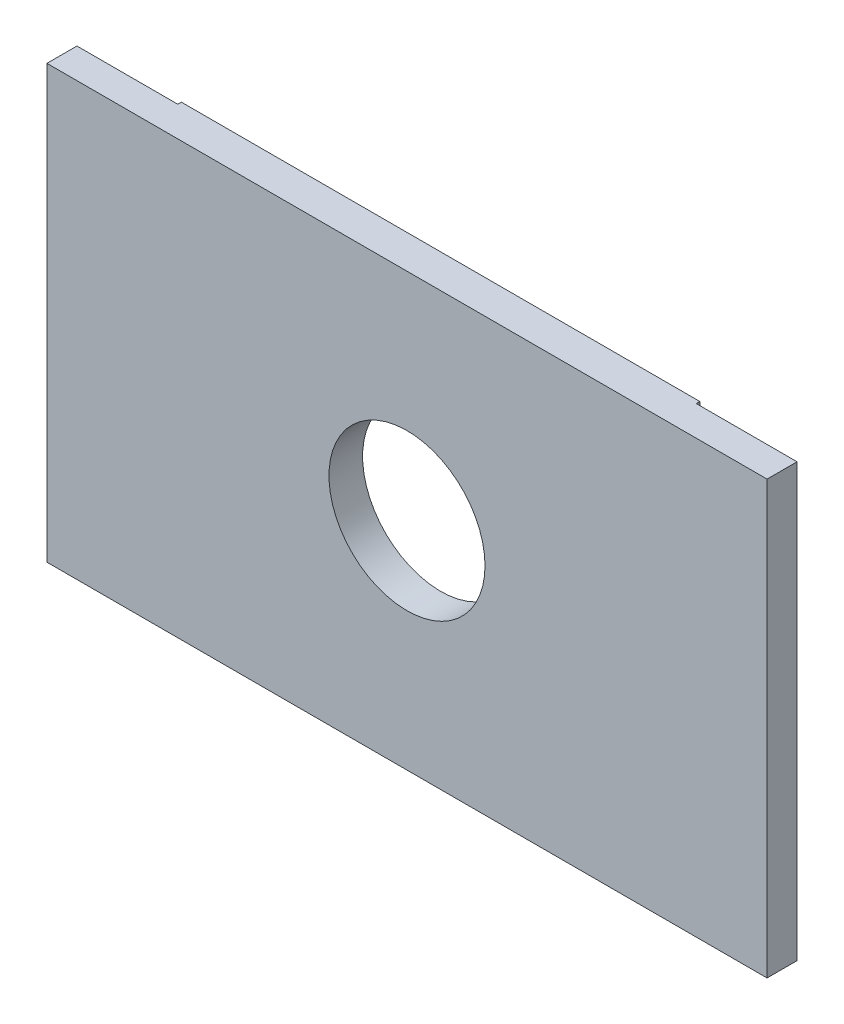
from build123d import *

# Parameters (mm, degrees)
SKETCH_1_W          = 300
SKETCH_1_H          = 180
EXTRUDE_1_DEPTH     = 14
SKETCH_2_W          = 42
SKETCH_2_H          = 180
CUT_EXTRUDE_1_DEPTH = 1.5
CUT_EXTRUDE_2_REACH = 177.488
SKETCH_3_R          = 32.5


with BuildPart() as part:
    # 草图1 → 凸台-拉伸1 (new body)
    with BuildSketch(Plane.XY):
        Rectangle(SKETCH_1_W, SKETCH_1_H)
    extrude(amount=EXTRUDE_1_DEPTH)

    # 草图2 → 切除-拉伸1 (cut)
    with BuildSketch(Plane(origin=(0, 0, 0), x_dir=(-1, 0, 0), z_dir=(0, 0, -1))):
        with Locations((129, 0)):
            Rectangle(SKETCH_2_W, SKETCH_2_H)
        with Locations((-129, 0)):
            Rectangle(SKETCH_2_W, SKETCH_2_H)
    extrude(amount=-CUT_EXTRUDE_1_DEPTH, mode=Mode.SUBTRACT)

    # 草图3 → 切除-拉伸2 (cut, up to next)
    with BuildSketch(Plane.XY.offset(14), mode=Mode.PRIVATE) as cut_extrude_2_sk1:
        Circle(SKETCH_3_R)
    cut_extrude_2_tool1 = extrude(cut_extrude_2_sk1.sketch, amount=-CUT_EXTRUDE_2_REACH, mode=Mode.PRIVATE) & part.part
    add(cut_extrude_2_tool1.solids().sort_by_distance((0, 0, 14))[0], mode=Mode.SUBTRACT)


solid = part.part
